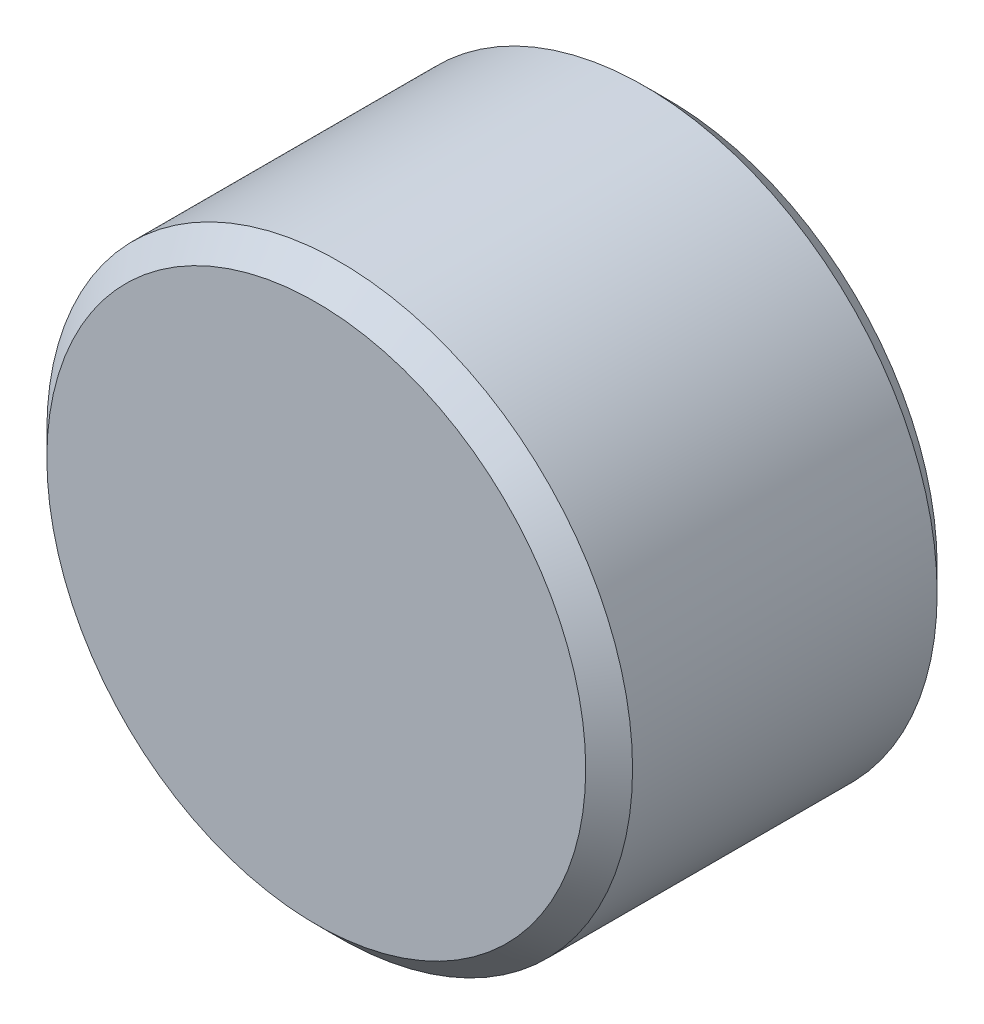
SolidWorks part; units mm, degrees
ref_plane "Front Plane" through (0, 0, 0) normal (0, 0, 1) x (1, 0, 0)
ref_plane "Top Plane" through (0, 0, 0) normal (0, 1, 0) x (1, 0, 0)
ref_plane "Right Plane" through (0, 0, 0) normal (1, 0, 0) x (0, 0, -1)
sketch "Sketch1" plane through (0, 0, 0) normal (0, 0, 1) x (1, 0, 0)
  circle A0 centre (0, 0) radius 25
  dimension "D1" = 50
extrude "Boss-Extrude1" add sketch "Sketch1" along normal blind 30
chamfer "Chamfer1" distance 2 angle 45 2 edges at (25, 0, 30) (25, 0, 0)
